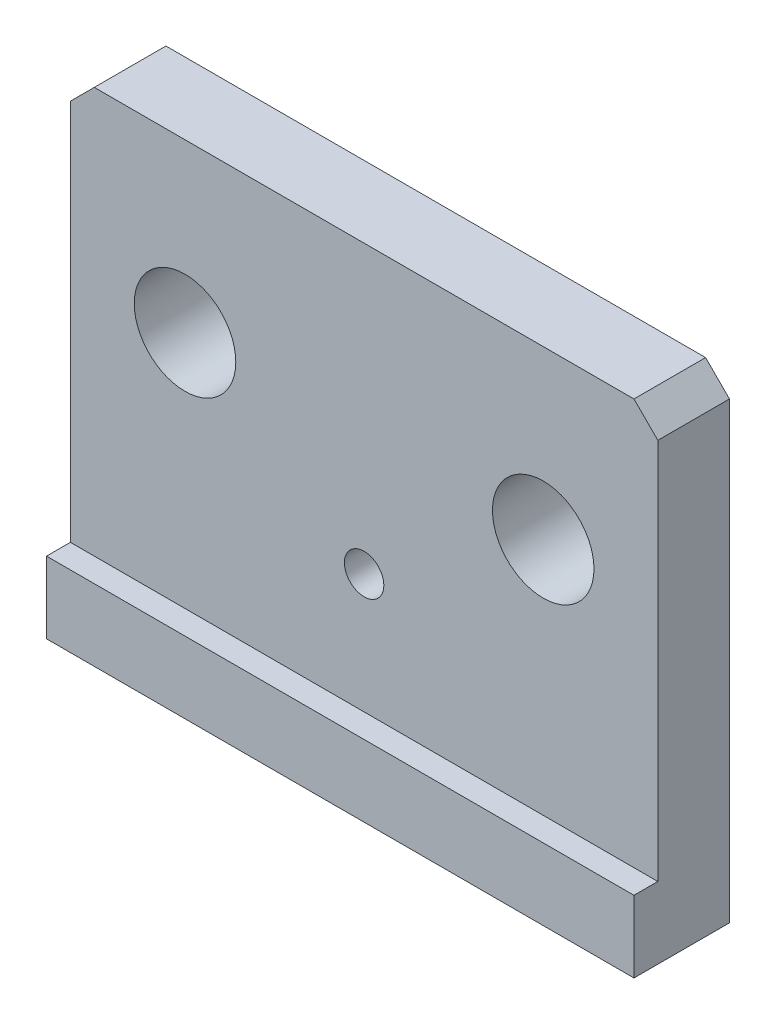
SolidWorks part; units mm, degrees
ref_plane "前视基准面" through (0, 0, 0) normal (0, 0, 1) x (1, 0, 0)
ref_plane "上视基准面" through (0, 0, 0) normal (0, 1, 0) x (1, 0, 0)
ref_plane "右视基准面" through (0, 0, 0) normal (1, 0, 0) x (0, 0, -1)
sketch "草图1" plane through (0, 0, 0) normal (0, 0, 1) x (1, 0, 0)
  line L1 (-24.6, 20) -> (24.6, 20)
  line L2 (-24.6, 20) -> (-24.6, -20)
  line L3 (-24.6, -20) -> (24.6, -20)
  line L4 (24.6, 20) -> (24.6, -20)
  line L5 (-24.6, 20) -> (24.6, -20) construction
  line L6 (-24.6, -20) -> (24.6, 20) construction
  point P0 (0, 0)
  dimension "D1" = 49.2
  dimension "D2" = 40
extrude "凸台-拉伸1" add sketch "草图1" along normal blind 8
hole_wizard "M4 螺纹孔1" positions "草图5" profile "草图4" tap size "M4" standard "Iso"
sketch "草图5" plane through (0, -20, 0) normal (0, -1, 0) x (-1, 0, 0)
  point P0 (12.7, -4)
  point P3 (-12.7, -4)
sketch "草图4" plane through (-12.7, -20, 4) normal (1, 0, 0) x (0, 0, -1)
  line L0 (0, 0) -> (0, 11.0914)
  line L1 (0, 11.0914) -> (1.65, 10.1)
  line L2 (1.65, 10.1) -> (1.65, 0)
  line L5 (1.65, 0) -> (0, 0)
  line L10 (0, 11.0914) -> (-1.65, 10.1) construction
  line L11 (0, -6.35) -> (0, 107.95) construction
  dimension "螺纹孔钻头直径" = 3.3
  dimension "螺纹孔钻头深度" = 10.1
  dimension "导头角度" = 118
cosmetic thread "孔螺蚊线1" parameters "D1"=8, "D2"=4
cosmetic thread "孔螺蚊线2" parameters "D1"=8, "D2"=4
chamfer "倒角1" distance 2 angle 45 2 edges at (24.6, 20, 4) (-24.6, 20, 4)
sketch "草图8" plane through (0, 0, 8) normal (0, 0, 1) x (1, 0, 0)
  line L0 (-24.6, -20) -> (24.6, -20) construction
  line L1 (-24.9686, 22.1981) -> (30.3043, 22.1981)
  line L2 (-24.9686, 22.1981) -> (-24.9686, -14)
  line L3 (-24.9686, -14) -> (30.3043, -14)
  line L4 (30.3043, 22.1981) -> (30.3043, -14)
  dimension "D1" = 6
extrude "切除-拉伸3" cut sketch "草图8" against normal blind 2
sketch "草图9" plane through (0, 0, 0) normal (0, 0, -1) x (-1, 0, 0)
  line L0 (0, 0) -> (0, 20) construction
  line L1 (-22.6, 20) -> (22.6, 20) construction
  line L2 (24.6, -20) -> (-24.6, -20) construction
  circle A0 centre (-15, 6) radius 4.25
  circle A1 centre (15, 6) radius 4.25
  dimension "D1" = 26
  dimension "D2" = 30
  dimension "D3" = 8.5
extrude "切除-拉伸4" cut sketch "草图9" against normal blind 25
hole_wizard "M4 螺纹孔2" positions "草图11" profile "草图10" tap size "M4" standard "Iso"
sketch "草图11" plane through (0, 0, 6) normal (0, 0, 1) x (1, 0, 0)
  line L0 (-24.6, -14) -> (24.6, -14) construction
  point P0 (0, -4)
  dimension "D1" = 10
sketch "草图10" plane through (0, -4, 6) normal (1, 0, 0) x (0, -1, 0)
  line L0 (0, 0) -> (0, 11.0914)
  line L1 (0, 11.0914) -> (1.65, 10.1)
  line L2 (1.65, 10.1) -> (1.65, 0)
  line L5 (1.65, 0) -> (0, 0)
  line L10 (0, 11.0914) -> (-1.65, 10.1) construction
  line L11 (0, -6.35) -> (0, 107.95) construction
  dimension "螺纹孔钻头直径" = 3.3
  dimension "螺纹孔钻头深度" = 10.1
  dimension "导头角度" = 118
cosmetic thread "孔螺蚊线3" parameters "D1"=6, "D2"=4
